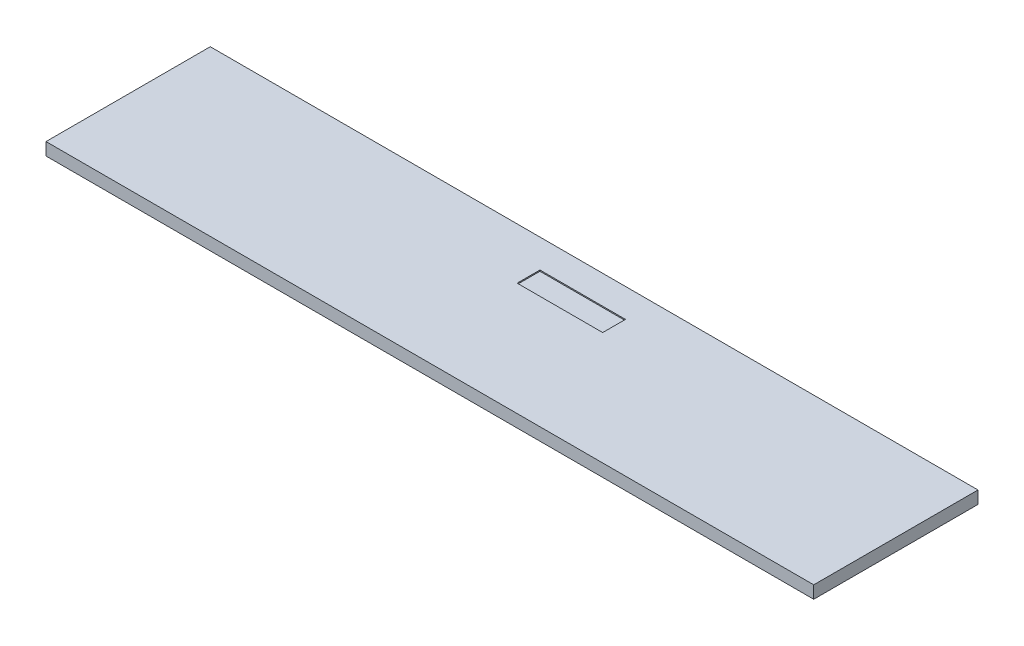
from build123d import *

# Parameters (mm, degrees)
SKETCH_1_W          = 1346
SKETCH_1_H          = 288
EXTRUDE_1_DEPTH     = 20
SHELL_1_T           = -2
SKETCH_2_W          = 1346
SKETCH_2_H          = 288
EXTRUDE_2_DEPTH     = 2
SKETCH_4_W          = 150
SKETCH_4_H          = 40
CUT_EXTRUDE_1_DEPTH = 2


with BuildPart() as part:
    # 草图1 → 凸台-拉伸1 (new body)
    with BuildSketch(Plane(origin=(0, 0, 0), x_dir=(1, 0, 0), z_dir=(0, 1, 0))):
        Rectangle(SKETCH_1_W, SKETCH_1_H)
    extrude(amount=-EXTRUDE_1_DEPTH)

    # 抽壳1
    shell_1_openings = [part.faces().sort_by_distance(p)[0] for p in [
        (0, -20, 0),
    ]]
    offset(amount=SHELL_1_T, openings=shell_1_openings, kind=Kind.INTERSECTION)

    # 草图2 → 凸台-拉伸2 (add)
    with BuildSketch(Plane.XZ.offset(20)):
        Rectangle(SKETCH_2_W, SKETCH_2_H)
    extrude(amount=EXTRUDE_2_DEPTH)

    # 草图4 → 切除-拉伸1 (cut)
    with BuildSketch(Plane(origin=(0, 0, 0), x_dir=(1, 0, 0), z_dir=(0, 1, 0))):
        with Locations((30, 74)):
            Rectangle(SKETCH_4_W, SKETCH_4_H)
    extrude(amount=-CUT_EXTRUDE_1_DEPTH, mode=Mode.SUBTRACT)


solid = part.part
